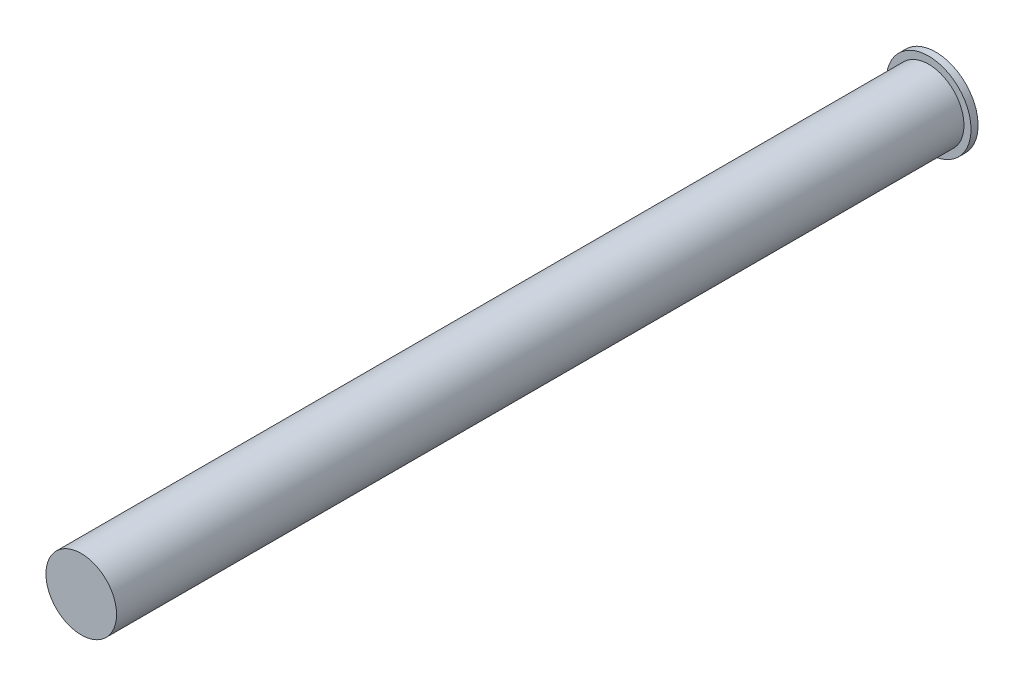
SolidWorks part; units mm, degrees
ref_plane "前视基准面" through (0, 0, 0) normal (0, 0, 1) x (1, 0, 0)
ref_plane "上视基准面" through (0, 0, 0) normal (0, 1, 0) x (1, 0, 0)
ref_plane "右视基准面" through (0, 0, 0) normal (1, 0, 0) x (0, 0, -1)
sketch "草图1" plane through (0, 0, 0) normal (0, 0, 1) x (1, 0, 0)
  circle A0 centre (0, 0) radius 5
  dimension "D1" = 10
extrude "凸台-拉伸1" add sketch "草图1" along normal blind 120
sketch "草图2" plane through (0, 0, 0) normal (0, 0, -1) x (-1, 0, 0)
  circle A0 centre (0, 0) radius 6
  dimension "D1" = 12
extrude "凸台-拉伸2" add sketch "草图2" along normal blind 1
